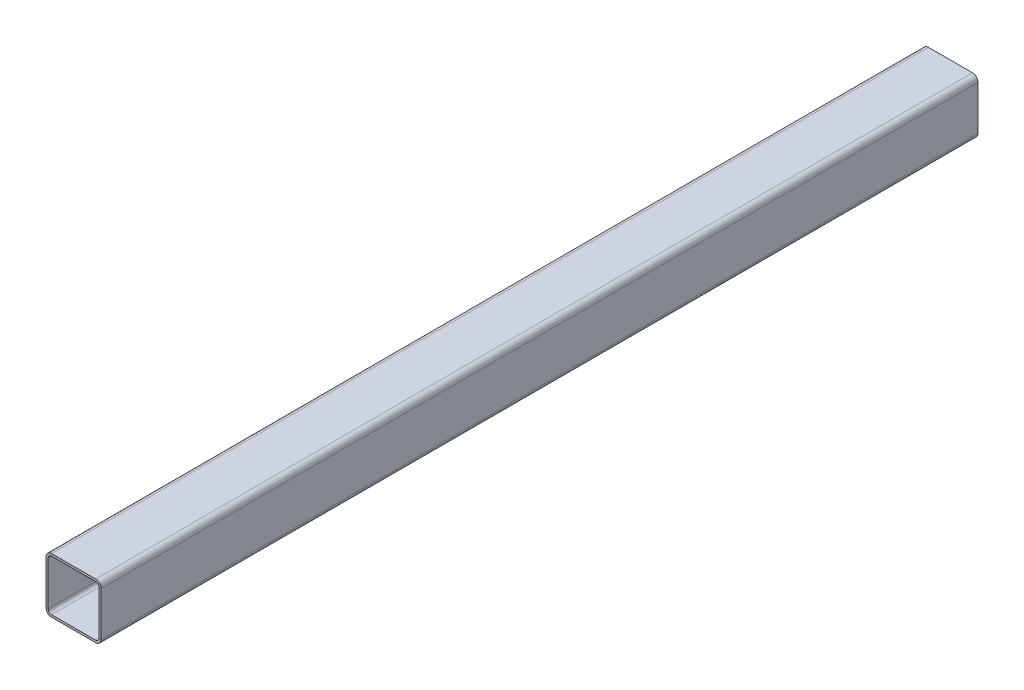
from build123d import *

# Parameters (mm, degrees)
BOSS_EXTRUDE1_DEPTH = 3180


with BuildPart() as part:
    # Sketch1 → Boss-Extrude1 (new body)
    with BuildSketch(Plane.XY):
        with BuildLine():
            Line((-80, 100), (80, 100))
            ThreePointArc((80, 100), (94.142135624, 94.142135624), (100, 80))
            Line((100, 80), (100, -80))
            ThreePointArc((100, -80), (94.142135624, -94.142135624), (80, -100))
            Line((80, -100), (-80, -100))
            ThreePointArc((-80, -100), (-94.142135624, -94.142135624), (-100, -80))
            Line((-100, -80), (-100, 80))
            ThreePointArc((-100, 80), (-94.142135624, 94.142135624), (-80, 100))
        make_face()
        with BuildLine():
            Line((-92, 80), (-92, -80))
            ThreePointArc((-92, -80), (-88.485281374, -88.485281374), (-80, -92))
            Line((-80, -92), (80, -92))
            ThreePointArc((80, -92), (88.485281374, -88.485281374), (92, -80))
            Line((92, -80), (92, 80))
            ThreePointArc((92, 80), (88.485281374, 88.485281374), (80, 92))
            Line((80, 92), (-80, 92))
            ThreePointArc((-80, 92), (-88.485281374, 88.485281374), (-92, 80))
        make_face(mode=Mode.SUBTRACT)
    extrude(amount=BOSS_EXTRUDE1_DEPTH)


solid = part.part
